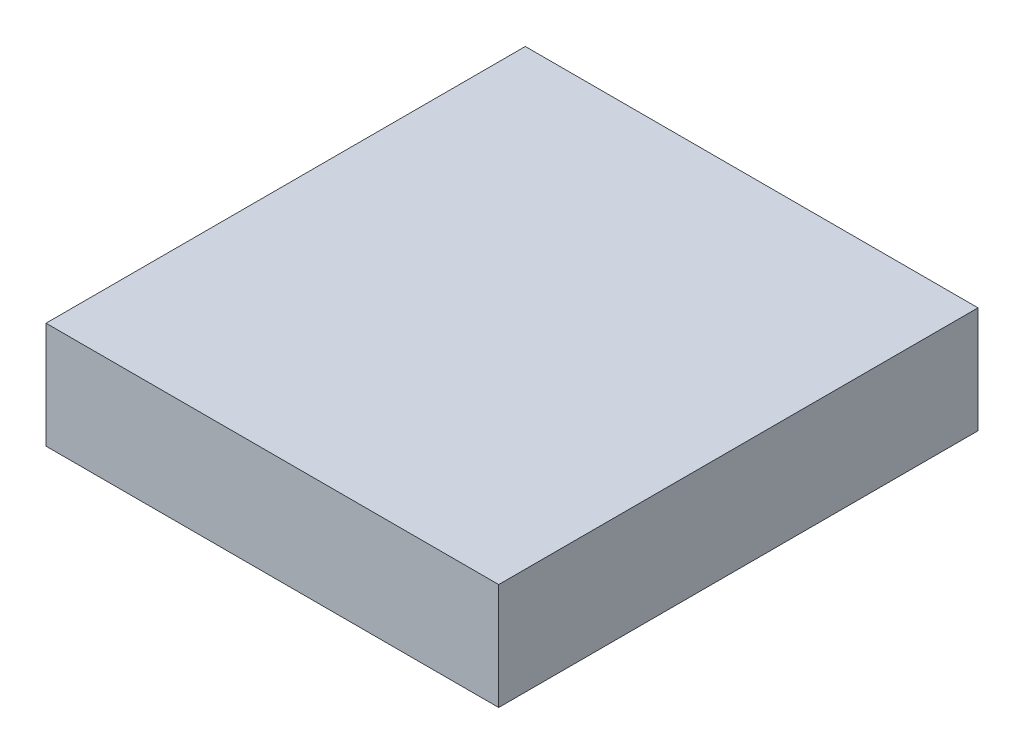
from build123d import *

# Parameters (mm, degrees)
SKETCH_1_W      = 170
SKETCH_1_H      = 180
EXTRUDE_1_DEPTH = 40


with BuildPart() as part:
    # 草图1 → 凸台-拉伸1 (new body)
    with BuildSketch(Plane(origin=(0, 0, 0), x_dir=(1, 0, 0), z_dir=(0, 1, 0))):
        Rectangle(SKETCH_1_W, SKETCH_1_H)
    extrude(amount=EXTRUDE_1_DEPTH)


solid = part.part
